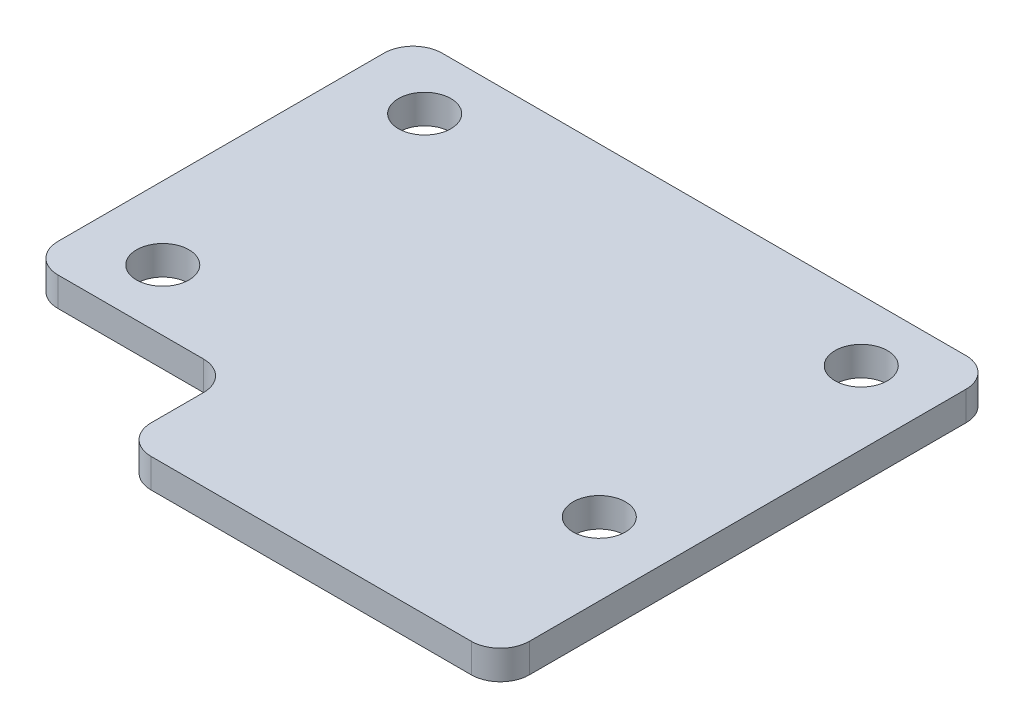
SolidWorks part; units mm, degrees
material "Q235"
ref_plane "Front Plane" through (0, 0, 0) normal (0, 0, 1) x (1, 0, 0)
ref_plane "Top Plane" through (0, 0, 0) normal (0, 1, 0) x (1, 0, 0)
ref_plane "Right Plane" through (0, 0, 0) normal (1, 0, 0) x (0, 0, -1)
sketch "Sketch2" plane through (0, 0, 0) normal (0, 1, 0) x (1, 0, 0)
  line L1 (-50, 42.5) -> (50, 42.5)
  line L2 (-50, 42.5) -> (-50, -42.5)
  line L3 (-50, -42.5) -> (50, -42.5)
  line L4 (50, 42.5) -> (50, -42.5)
  line L5 (-50, 42.5) -> (50, -42.5) construction
  line L6 (-50, -42.5) -> (50, 42.5) construction
  point P0 (0, 0)
  dimension "D1" = 100
  dimension "D2" = 85
extrude "Boss-Extrude1" add sketch "Sketch2" along normal blind 5
hole_wizard "M8 Clearance Hole1" positions "Sketch4" profile "Sketch5" hole size "M8" standard "GB" end condition through all
sketch "Sketch4" plane through (0, 5, 0) normal (0, 1, 0) x (1, 0, 0)
  line L0 (0, 42.5) -> (0, 36.6866) construction
  line L1 (50, 42.5) -> (-50, 42.5) construction
  point P0 (-37.5, 32)
  point P2 (37.5, 32)
  point P4 (37.5, -13)
  point P6 (-37.5, -13)
  dimension "D1" = 75
  dimension "D2" = 45
  dimension "D3" = 10.5
sketch "Sketch5" plane through (-37.5, 5, -32) normal (1, 0, 0) x (0, 0, 1)
  line L0 (0, 0) -> (0, 5)
  line L1 (0, 5) -> (4.5, 5)
  line L2 (4.5, 5) -> (4.5, 0)
  line L5 (4.5, 0) -> (0, 0)
  line L11 (0, -6.35) -> (0, 107.95) construction
  dimension "通孔孔直径" = 9
  dimension "通孔孔深度" = 5
fillet "Fillet1" radius 5 3 edges at (50, 2.5, 42.5) (50, 2.5, -42.5) (-50, 2.5, -42.5)
sketch "Sketch7" plane through (0, 5, 0) normal (0, 1, 0) x (1, 0, 0)
  line L1 (-50, -42.5) -> (-15, -42.5)
  line L2 (-50, -42.5) -> (-50, -23.5)
  line L3 (-50, -23.5) -> (-15, -23.5)
  line L4 (-15, -42.5) -> (-15, -23.5)
  circle A0 centre (-37.5, -13) radius 4.5 construction
  dimension "D1" = 10.5
  dimension "D2" = 35
extrude "Cut-Extrude1" cut sketch "Sketch7" against normal blind 5
fillet "Fillet2" radius 5 3 edges at (-15, 2.5, 42.5) (-15, 2.5, 23.5) (-50, 2.5, 23.5)
